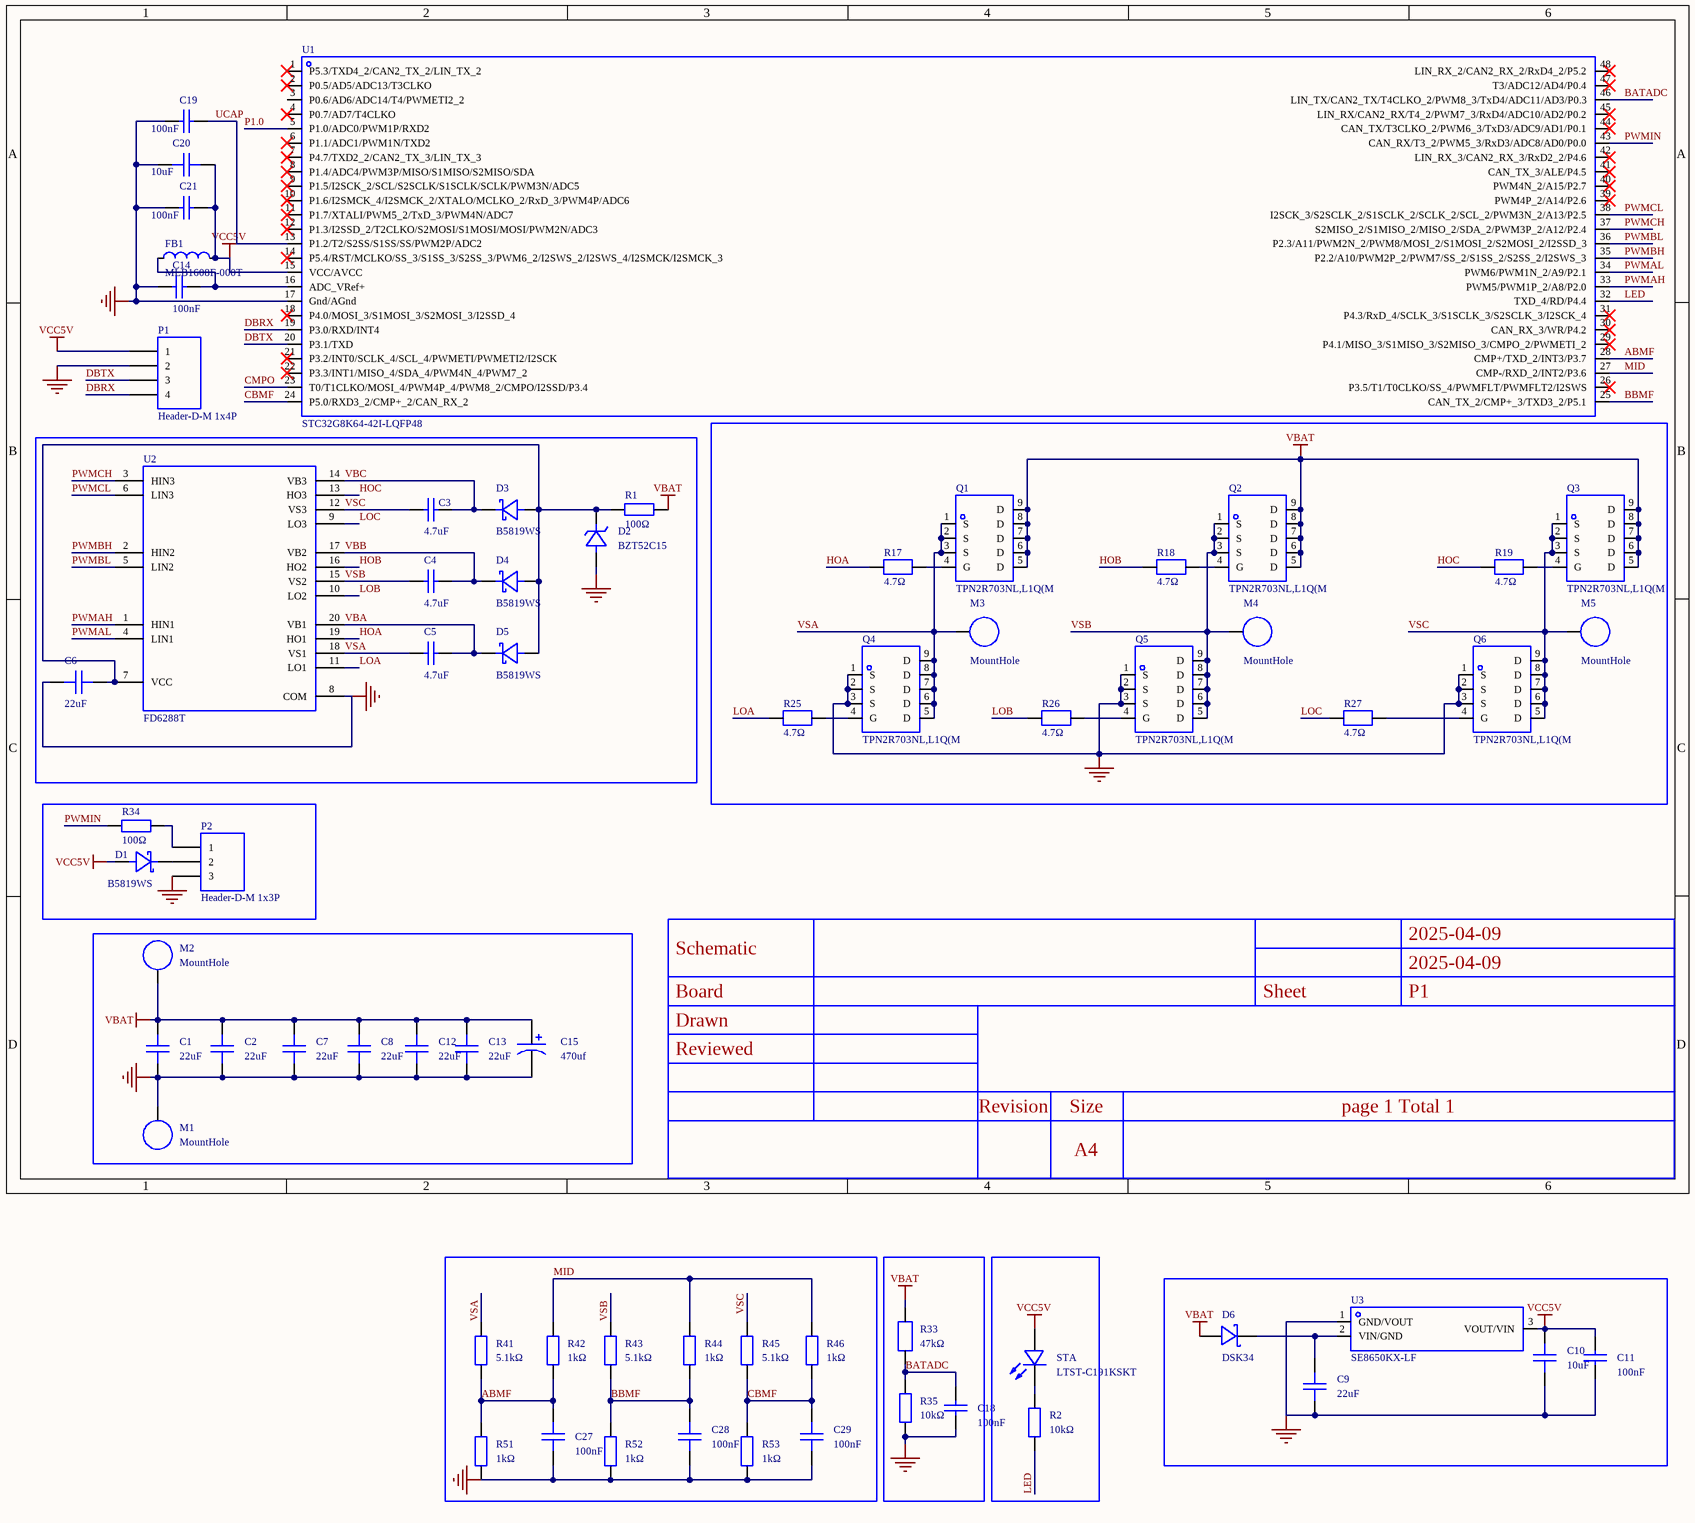
[diagram p0: MISC52085-3.schdoc]
# Altium project MISC52085-2.PrjPcb
1 sheet, 66 parts. Net scope: global (net labels, ports and power ports of the same name join across sheets).
Board file: MISC52085.pcbdoc

## Sheet MISC52085-3.schdoc
size 297 x 209 mm; Version: V1.0; @Project Name: MISC52085; @Page Count: 1; @Update Date: 2025-04-09; @Create Date: 2025-04-09; @Schematic Name: MISC52085; @Page No: 1; @Create Time: 14:04:51; @Update Time: 14:05:14; @Board Name: MISC52085

### Parts
C1  22uF  [C0805]
C2  22uF  [C0805]
C3  4.7uF  [C0805]
C4  4.7uF  [C0805]
C5  4.7uF  [C0805]
C6  22uF  [C0805]
C7  22uF  [C0805]
C8  22uF  [C0805]
C9  22uF  [C0805]
C10  10uF  [C0603]
C11  100nF  [C0603]
C12  22uF  [C0805]
C13  22uF  [C0805]
C14  100nF  [C0603]
C15  470uf  [焊盘]
C18  100nF  [C0603]
C19  100nF  [C0603]
C20  10uF  [C0603]
C21  100nF  [C0603]
C27  100nF  [C0402]
C28  100nF  [C0402]
C29  100nF  [C0402]
D1  B5819WS  [SOD-323_L1.7-W1.3-LS2.5-FD]
D2  BZT52C15  [SOD-123_L2.7-W1.6-LS3.7-RD]
D3  B5819WS  [SOD-323_L1.7-W1.3-LS2.5-FD]
D4  B5819WS  [SOD-323_L1.7-W1.3-LS2.5-FD]
D5  B5819WS  [SOD-323_L1.7-W1.3-LS2.5-FD]
D6  DSK34  [SOD-123_L2.8-W1.8-LS3.7-RD]
FB1  MLB1608F-000T  [L0603]
M1  MountHole  [3*4焊盘]
M2  MountHole  [3*4焊盘]
M3  MountHole  [3*4焊盘]
M4  MountHole  [3*4焊盘]
M5  MountHole  [3*4焊盘]
P1  Header-D-M 1x4P  [调试端口2.54_1X4]
P2  Header-D-M 1x3P  [3P]
Q1  TPN2R703NL,L1Q(M  [TSON-8_L3.1-W3.1-P0.65-LS3.3-BL-EP]
Q2  TPN2R703NL,L1Q(M  [TSON-8_L3.1-W3.1-P0.65-LS3.3-BL-EP]
Q3  TPN2R703NL,L1Q(M  [TSON-8_L3.1-W3.1-P0.65-LS3.3-BL-EP]
Q4  TPN2R703NL,L1Q(M  [TSON-8_L3.1-W3.1-P0.65-LS3.3-BL-EP]
Q5  TPN2R703NL,L1Q(M  [TSON-8_L3.1-W3.1-P0.65-LS3.3-BL-EP]
Q6  TPN2R703NL,L1Q(M  [TSON-8_L3.1-W3.1-P0.65-LS3.3-BL-EP]
R1  100Ω  [R0603]
R2  10kΩ  [R0603]
R17  4.7Ω  [R0603]
R18  4.7Ω  [R0603]
R19  4.7Ω  [R0603]
R25  4.7Ω  [R0603]
R26  4.7Ω  [R0603]
R27  4.7Ω  [R0603]
R33  47kΩ  [R0603]
R34  100Ω  [R0603]
R35  10kΩ  [R0603]
R41  5.1kΩ  [R0603]
R42  1kΩ  [R0603]
R43  5.1kΩ  [R0603]
R44  1kΩ  [R0603]
R45  5.1kΩ  [R0603]
R46  1kΩ  [R0603]
R51  1kΩ  [R0603]
R52  1kΩ  [R0603]
R53  1kΩ  [R0603]
STA  LTST-C191KSKT  [LED0603-RD-YELLOW]
U1  STC32G8K64-42I-LQFP48  [LQFP-48_L7.0-W7.0-P0.50-LS9.0-BL]
U2  FD6288T  [TSSOP-20_L6.5-W4.4-P0.65-LS6.4-BL]
U3  SE8650KX-LF  [SOT-89-3_L4.3-W2.3-P1.50-LS4.3-BR]

### Nets
GND: C1.1 C2.1 C6.1 C7.1 C8.1 C9.1 C10.1 C11.1 C12.1 C13.1 C14.1 C15.2 C18.1 C19.1 C20.1 C21.1 C27.1 C28.1 C29.1 D2.2(A) M1.1 P1.2 P2.3 Q4.1(S) Q4.2(S) Q4.3(S) Q5.1(S) Q5.2(S) Q5.3(S) Q6.1(S) Q6.2(S) Q6.3(S) R35.1 R51.1 R52.1 R53.1 U1.17(Gnd/AGnd) U2.8(COM) U3.1(GND/VOUT)
VBAT: C1.2 C2.2 C7.2 C8.2 C12.2 C13.2 C15.1 D6.2(A) M2.1 Q1.5(D) Q1.6(D) Q1.7(D) Q1.8(D) Q1.9(D) Q2.5(D) Q2.6(D) Q2.7(D) Q2.8(D) Q2.9(D) Q3.5(D) Q3.6(D) Q3.7(D) Q3.8(D) Q3.9(D) R1.2 R33.2
VCC5V: C10.2 C11.2 C20.2 C21.2 D1.1(A) FB1.2 P1.1 STA.2(+) U1.15(VCC/AVCC) U3.3(VOUT/VIN)
ABMF: C27.2 R41.1 R42.1 R51.2 U1.28(CMP+/TXD_2/INT3/P3.7)
BATADC: C18.2 R33.1 R35.2 U1.46(LIN_TX/CAN2_TX/T4CLKO_2/PWM8_3/TxD4/ADC11/AD3/P0.3)
BBMF: C28.2 R43.1 R44.1 R52.2 U1.25(CAN_TX_2/CMP+_3/TXD3_2/P5.1)
CBMF: C29.2 R45.1 R46.1 R53.2 U1.24(P5.0/RXD3_2/CMP+_2/CAN_RX_2)
CMPO: U1.23(T0/T1CLKO/MOSI_4/PWM4P_4/PWM8_2/CMPO/I2SSD/P3.4)
DBRX: P1.4 U1.19(P3.0/RXD/INT4)
DBTX: P1.3 U1.20(P3.1/TXD)
HOA: R17.1 U2.19(HO1)
HOB: R18.1 U2.16(HO2)
HOC: R19.1 U2.13(HO3)
LED: R2.1 U1.32(TXD_4/RD/P4.4)
LOA: R25.1 U2.11(LO1)
LOB: R26.1 U2.10(LO2)
LOC: R27.1 U2.9(LO3)
MID: R42.2 R44.2 R46.2 U1.27(CMP-/RXD_2/INT2/P3.6)
P1.0: U1.5(P1.0/ADC0/PWM1P/RXD2)
PWMAH: U1.33(PWM5/PWM1P_2/A8/P2.0) U2.1(HIN1)
PWMAL: U1.34(PWM6/PWM1N_2/A9/P2.1) U2.4(LIN1)
PWMBH: U1.35(P2.2/A10/PWM2P_2/PWM7/SS_2/S1SS_2/S2SS_2/I2SWS_3) U2.2(HIN2)
PWMBL: U1.36(P2.3/A11/PWM2N_2/PWM8/MOSI_2/S1MOSI_2/S2MOSI_2/I2SSD_3) U2.5(LIN2)
PWMCH: U1.37(S2MISO_2/S1MISO_2/MISO_2/SDA_2/PWM3P_2/A12/P2.4) U2.3(HIN3)
PWMCL: U1.38(I2SCK_3/S2SCLK_2/S1SCLK_2/SCLK_2/SCL_2/PWM3N_2/A13/P2.5) U2.6(LIN3)
PWMIN: R34.1 U1.43(CAN_RX/T3_2/PWM5_3/RxD3/ADC8/AD0/P0.0)
UCAP: C19.2 U1.13(P1.2/T2/S2SS/S1SS/SS/PWM2P/ADC2)
VBA: C5.2 D5.2(K) U2.20(VB1)
VBB: C4.2 D4.2(K) U2.17(VB2)
VBC: C3.2 D3.2(K) U2.14(VB3)
VSA: C5.1 M3.1 Q1.1(S) Q1.2(S) Q1.3(S) Q4.5(D) Q4.6(D) Q4.7(D) Q4.8(D) Q4.9(D) R41.2 U2.18(VS1)
VSB: C4.1 M4.1 Q2.1(S) Q2.2(S) Q2.3(S) Q5.5(D) Q5.6(D) Q5.7(D) Q5.8(D) Q5.9(D) R43.2 U2.15(VS2)
VSC: C3.1 M5.1 Q3.1(S) Q3.2(S) Q3.3(S) Q6.5(D) Q6.6(D) Q6.7(D) Q6.8(D) Q6.9(D) R45.2 U2.12(VS3)
NetC6_2: C6.2 D2.1(K) D3.1(A) D4.1(A) D5.1(A) R1.1 U2.7(VCC)
NetC9_2: C9.2 D6.1(K) U3.2(VIN/GND)
NetC14_2: C14.2 FB1.1 U1.16(ADC_VRef+)
NetD1_2: D1.2(K) P2.2
NetP2_1: P2.1 R34.2
NetQ1_4: Q1.4(G) R17.2
NetQ2_4: Q2.4(G) R18.2
NetQ3_4: Q3.4(G) R19.2
NetQ4_4: Q4.4(G) R25.2
NetQ5_4: Q5.4(G) R26.2
NetQ6_4: Q6.4(G) R27.2
NetR2_2: R2.2 STA.1(-)

Not connected (* = marked no-connect by the designer): U1 1(P5.3/TXD4_2/CAN2_TX_2/LIN_TX_2)* 2(P0.5/AD5/ADC13/T3CLKO)* 3(P0.6/AD6/ADC14/T4/PWMETI2_2) 4(P0.7/AD7/T4CLKO)* 6(P1.1/ADC1/PWM1N/TXD2)* 7(P4.7/TXD2_2/CAN2_TX_3/LIN_TX_3)* 8(P1.4/ADC4/PWM3P/MISO/S1MISO/S2MISO/SDA)* 9(P1.5/I2SCK_2/SCL/S2SCLK/S1SCLK/SCLK/PWM3N/ADC5)* 10(P1.6/I2SMCK_4/I2SMCK_2/XTALO/MCLKO_2/RxD_3/PWM4P/ADC6)* 11(P1.7/XTALI/PWM5_2/TxD_3/PWM4N/ADC7)* 12(P1.3/I2SSD_2/T2CLKO/S2MOSI/S1MOSI/MOSI/PWM2N/ADC3)* 14(P5.4/RST/MCLKO/SS_3/S1SS_3/S2SS_3/PWM6_2/I2SWS_2/I2SWS_4/I2SMCK/I2SMCK_3)* 18(P4.0/MOSI_3/S1MOSI_3/S2MOSI_3/I2SSD_4)* 21(P3.2/INT0/SCLK_4/SCL_4/PWMETI/PWMETI2/I2SCK)* 22(P3.3/INT1/MISO_4/SDA_4/PWM4N_4/PWM7_2)* 26(P3.5/T1/T0CLKO/SS_4/PWMFLT/PWMFLT2/I2SWS)* 29(P4.1/MISO_3/S1MISO_3/S2MISO_3/CMPO_2/PWMETI_2)* 30(CAN_RX_3/WR/P4.2)* 31(P4.3/RxD_4/SCLK_3/S1SCLK_3/S2SCLK_3/I2SCK_4)* 39(PWM4P_2/A14/P2.6)* 40(PWM4N_2/A15/P2.7)* 41(CAN_TX_3/ALE/P4.5)* 42(LIN_RX_3/CAN2_RX_3/RxD2_2/P4.6)* 44(CAN_TX/T3CLKO_2/PWM6_3/TxD3/ADC9/AD1/P0.1)* 45(LIN_RX/CAN2_RX/T4_2/PWM7_3/RxD4/ADC10/AD2/P0.2)* 47(T3/ADC12/AD4/P0.4)* 48(LIN_RX_2/CAN2_RX_2/RxD4_2/P5.2)*

### Notes on the sheet
- 2025-04-09
- Schematic
- Board
- Sheet
- P1
- Drawn
- Reviewed
- Revision
- Size
- A4
- page 1 Total 1

### Library data of the parts
C1 C2 C6-C9 C12 C13 = CL21A226MAQNNNE: Capacitance:22uF;Tolerance:±20%;Rated voltage:25V;Dielectric (temp. coefficient):X5R;; Manufacturer: SAMSUNG(三星); AddInBom: yes; ModelId: 1ba041120af144c991958decab20d241; ModelName: C0805_L2.0-W1.3-H1.3; ModelTransform: 78.74,51.181,0,0,0,0,0,0.0005,0; Tolerance: ±20%; Voltage Rated: 25V; Temperature Coefficient: X5R; Symbol: CL21A226MAQNNNE; Device: CL21A226MAQNNNE; LCSC Part Name: 22uF ±20% 25V; SupplierPart: C45783; ManufacturerPart: CL21A226MAQNNNE; Supplier Footprint: 0805; JLCPCB Part Class: Basic library; Datasheet: https://atta.szlcsc.com/upload/public/pdf/source/20160218/1457707763339.pdf; Supplier: LCSC; ConvertToPcb: yes; FootprintName: C0805; Value: 22uF
C3-C5 = CL21A475KAQNNNE: Capacitance:4.7uF;Tolerance:±10%;Rated voltage:25V;Dielectric (temp. coefficient):X5R;; Manufacturer: SAMSUNG(三星); AddInBom: yes; ModelId: 1ba041120af144c991958decab20d241; ModelName: C0805_L2.0-W1.3-H1.3; ModelTransform: 78.74,51.181,0,0,0,0,0,0.0005,0; Tolerance: ±10%; Voltage Rated: 25V; Temperature Coefficient: X5R; Symbol: CL21A475KAQNNNE; Device: CL21A475KAQNNNE; LCSC Part Name: 4.7uF ±10% 25V; SupplierPart: C1779; ManufacturerPart: CL21A475KAQNNNE; Supplier Footprint: 0805; JLCPCB Part Class: Basic library; Datasheet: https://atta.szlcsc.com/upload/public/pdf/source/20160218/1457707763339.pdf; Supplier: LCSC; ConvertToPcb: yes; FootprintName: C0805; Value: 4.7uF
C10 C20 = CGA0603X5R106K100JT: Capacitance:10uF;Tolerance:±10%;Rated voltage:10V;Temperature coefficient:X5R;; Manufacturer: HRE(芯声); AddInBom: yes; ModelId: ac125912035d415993ca9572d50418b1; ModelName: C0603_L1.6-W0.8-H0.8; ModelTransform: 62.992,31.496,0,0,0,0,0,0,0; Tolerance: ±10%; Voltage Rating: 10V; Temperature Coefficient: X5R; Symbol: CGA0603X5R106K100JT; Device: CGA0603X5R106K100JT; LCSC Part Name: 10uF ±10% 10V; SupplierPart: C6119842; ManufacturerPart: CGA0603X5R106K100JT; Supplier Footprint: 0603; JLCPCB Part Class: Extended library; Supplier: LCSC; ConvertToPcb: yes; FootprintName: C0603; Value: 10uF
C11 C14 C18 C19 C21 = CL10B104KO8NNNC: Capacitance:100nF;Tolerance:±10%;Rated voltage:16V;Dielectric (temp. coefficient):X7R;; Manufacturer: SAMSUNG(三星); AddInBom: yes; ModelId: ac125912035d415993ca9572d50418b1; ModelName: C0603_L1.6-W0.8-H0.8; ModelTransform: 62.992,31.496,0,0,0,0,0,0,0; Tolerance: ±10%; Voltage Rated: 16V; Temperature Coefficient: X7R; Symbol: CL10B104KO8NNNC; Device: CL10B104KO8NNNC; LCSC Part Name: 100nF ±10% 16V; SupplierPart: C66501; ManufacturerPart: CL10B104KO8NNNC; Supplier Footprint: 0603; JLCPCB Part Class: Extended library; Datasheet: https://atta.szlcsc.com/upload/public/pdf/source/20160218/1457707763339.pdf; Supplier: LCSC; ConvertToPcb: yes; FootprintName: C0603; Value: 100nF
C15 = 470uf: ConvertToPcb: yes; Device: 470uf; AddInBom: yes; SymbolName: 470uf
C27-C29 = CL05B104KO5NNNC: Capacitance:100nF;Tolerance:±10%;Rated voltage:16V;Dielectric (temp. coefficient):X7R;; Manufacturer: SAMSUNG(三星); AddInBom: yes; ModelId: 36a51122f27c49738f86b3bfa98863e0; ModelName: C0402_L1.0-W0.5-H0.5; ModelTransform: 39.37,19.685,0,0,0,0,0,0,0; Tolerance: ±10%; Voltage Rated: 16V; Temperature Coefficient: X7R; Symbol: CL05B104KO5NNNC; Device: CL05B104KO5NNNC; LCSC Part Name: 100nF ±10% 16V; SupplierPart: C1525; ManufacturerPart: CL05B104KO5NNNC; Supplier Footprint: 0402; JLCPCB Part Class: Basic library; Datasheet: https://atta.szlcsc.com/upload/public/pdf/source/20160218/1457707763339.pdf; Supplier: LCSC; ConvertToPcb: yes; FootprintName: C0402; Value: 100nF
D1 D3-D5 = B5819WS_C7420331: Diode configuration:Single;Forward voltage(Vf):600mV@1.0A;DC reverse voltage(Vr):40V;Rectified current:1A;; Manufacturer: 宏迦橙; AddInBom: yes; ModelId: 0f2f330c645944df9245ac3c3fec3456; ModelTransform: 98.425,49.2125,0,180,0,0,0,0,0; Diode Configuration: Single; Reverse Voltage (Vr): 40V; Rectified Current: 1A; Reverse Leakage Current (Ir): 1mA@40V; Symbol: B5819WS_C7420331; Device: B5819WS_C7420331; LCSC Part Name: 电压:40V 电流:1A; SupplierPart: C7420331; ManufacturerPart: B5819WS; Supplier Footprint: SOD-323; JLCPCB Part Class: Extended library; Datasheet: https://atta.szlcsc.com/upload/public/pdf/source/20230828/03CA0F4F90DAE368A7153B7B5E4D0651.pdf; Supplier: LCSC; ConvertToPcb: yes; FootprintName: SOD-323_L1.7-W1.3-LS2.5-FD; ModelName: SOD-323_L1.7-W1.3-LS2.5-FD; Forward Voltage (Vf@If): 600mV@1.0A
D2 = BZT52C15_C19077412: Diode configuration:Single;Zener voltage (nominal):15V;Zener voltage (range):14.25V~15.75V;Power dissipation(Pd):500mW;; Manufacturer: 宏嘉诚; AddInBom: yes; ModelId: ad7e39f9e5534b3c96ffdc5532ebb493; ModelName: SOD-123_L2.7-W1.6-H1.4-LS3.7; ModelTransform: 146.026,62.992,0,180,0,0,0.0005,0,0; Diode Configuration: Single; Zener Voltage(Nom): 15V; Reverse Leakage Current (Ir): 100nA@10.5V; Pd - Power Dissipation(Pd): 500mW; Impedance(Zzt): 40Ω; Symbol: BZT52C15_C19077412; Device: BZT52C15_C19077412; LCSC Part Name: BZT52C15; SupplierPart: C19077412; ManufacturerPart: BZT52C15; Supplier Footprint: SOD-123; JLCPCB Part Class: Extended library; Datasheet: https://atta.szlcsc.com/upload/public/pdf/source/20250106/E12AA82D484C9C66E469D005F460C1F7.pdf; Supplier: LCSC; ConvertToPcb: yes; FootprintName: SOD-123_L2.7-W1.6-LS3.7-RD; Zener Voltage(Range): 14.25V~15.75V
D6 = DSK34_C41029: Diode configuration:Single;Forward voltage(Vf):550mV@3A;DC reverse voltage(Vr):40V;Rectified current:3A;; Manufacturer: MDD(辰达半导体); AddInBom: yes; ModelId: 7884390a25fb4c08947731ebfba7e3f8; ModelTransform: 144.8816,62.992,0,0,0,0,0,0,0; Diode Configuration: Single; Reverse Voltage (Vr): 40V; Rectified Current: 3A; Reverse Leakage Current (Ir): 500uA@40V; Symbol: DSK34; Device: DSK34_C41029; LCSC Part Name: 电压:40V 电流:3A; SupplierPart: C41029; ManufacturerPart: DSK34; Supplier Footprint: SOD-123FL; JLCPCB Part Class: Extended library; Datasheet: https://atta.szlcsc.com/upload/public/pdf/source/20240710/931B7979AEEE628A0AE48522F9F6A0BB.pdf; Supplier: LCSC; ConvertToPcb: yes; FootprintName: SOD-123_L2.8-W1.8-LS3.7-RD; ModelName: SOD-123_L2.8-W1.8-LS3.7-RD; Forward Voltage (Vf@If): 550mV@3A
FB1 = MLB1608F-000T: Impedance@frequency:0Ω@100MHz;Tolerance:±25%;DC resistance(DCR):-;; Manufacturer: MetalLions(美铼); AddInBom: yes; ModelId: 2bc5ec593d464d6ba9807aec0b5673c2; ModelName: L0603_L1.6-W0.8-H0.5_BEAD; ModelTransform: 62.992,31.496,0,180,0,0,0.094,0.629,0; Tolerance: ±25%; Number of Circuits: 1; Symbol: MLB1608F-000T; Device: MLB1608F-000T; LCSC Part Name: 单路 0603磁珠 阻抗0Ω@100MHz; SupplierPart: C2844549; ManufacturerPart: MLB1608F-000T; Supplier Footprint: 0603; JLCPCB Part Class: Extended library; Datasheet: https://atta.szlcsc.com/upload/public/pdf/source/20230602/7F9B6FFD64AF4C161BE293D8440B9AF6.pdf; Supplier: LCSC; ConvertToPcb: yes; FootprintName: L0603; Impedance @ Frequency: 0Ω@100MHz; DC Resistance(DCR): -; Current Rating: -
M1-M5 = MountHole: Mounting hole; AddInBom: yes; Device: MountHole; Footprint Name: M3-MountHole-Plated-D6; ConvertToPcb: yes; SymbolName: MountHole
P1 = Header-D-M 1x4P: 1x4pin, through-hole, pin header; AddInBom: yes; Device: Header-D-M 1x4P; Revision: V1.0; Value: Header-D-M 1x4P; Footprint Name: HDR1X4-M; ConvertToPcb: yes; SymbolName: Header-D-M 1x4P
P2 = Header-D-M 1x3P: 1x3pin, through-hole, pin header; AddInBom: yes; Device: Header-D-M 1x3P; Revision: V1.0; Value: Header-D-M 1x3P; Footprint Name: HDR1X3-M; ConvertToPcb: yes; SymbolName: Header-D-M 1x3P
Q1-Q6 = TPN2R703NL,L1Q(M: Type:1 N-channel;Drain-source voltage(Vdss):30V;Continuous drain current(Id):-;On-resistance(RDS(on)@Vgs,Id):3.3mΩ@4.5V,22.5A;Power:42W;Threshold voltage(Vgs(th)@Id):1.3V@0.3mA;; Manufacturer: TOSHIBA(东芝); AddInBom: yes; ModelId: 054ae61349db4ab4a59bf8617c283080; ModelName: TSON-8_L3.1-W3.1-H0.9-P0.65-LS3.3-BL-EP; ModelTransform: 129.921,122.8344,0,90,0,0,0,0,0; Drain Source Voltage (Vdss): 30V; Power Dissipation (Pd): 42W; Input Capacitance (Ciss@Vds): 1.6nF@15V; Reverse Transfer Capacitance (Crss@Vds): 53pF@15V; Symbol: TPN2R703NL,L1Q(M; Device: TPN2R703NL,L1Q(M; LCSC Part Name: TPN2R703NL,L1Q(M; SupplierPart: C5307666; ManufacturerPart: TPN2R703NL,L1Q(M; Supplier Footprint: TSON-8; JLCPCB Part Class: Extended library; Datasheet: https://atta.szlcsc.com/upload/public/pdf/source/20221207/F3F28B90115C5E074AC0CD2ED28456D7.pdf; Supplier: LCSC; ConvertToPcb: yes; FootprintName: TSON-8_L3.1-W3.1-P0.65-LS3.3-BL-EP; Type: 1 N-channel; Continuous Drain Current (Id): -; Drain Source On Resistance (RDS(on)@Vgs,Id): 3.3mΩ@4.5V,22.5A; Gate Threshold Voltage (Vgs(th)@Id): 1.3V@0.3mA; Total Gate Charge (Qg@Vgs): -; Operating Temperature: -; Configuration: -
R1 R34 = 0603WAF1000T5E: Resistor type:Thick film resistor;Resistance:100Ω;Tolerance:±1%;Power:100mW;Max working voltage:75V;Temperature coefficient:±200ppm/℃;; Manufacturer: UNI-ROYAL(厚声); AddInBom: yes; ModelId: fc143cca1e79419f9cd78b61e9279f08; ModelTransform: 31.8897,63.7794,0,90,0,0,0,0,0; Tolerance: ±1%; Power(Watts): 100mW; Overload Voltage (Max): 75V; Symbol: 0603WAF1000T5E; Device: 0603WAF1000T5E; LCSC Part Name: 100Ω ±1% 100mW 厚膜电阻; SupplierPart: C22775; ManufacturerPart: 0603WAF1000T5E; Supplier Footprint: 0603; JLCPCB Part Class: Basic library; Datasheet: https://atta.szlcsc.com/upload/public/pdf/source/20200306/C422600_1E6D84923E4A46A82E41ADD87F860B5C.pdf; Supplier: LCSC; ConvertToPcb: yes; FootprintName: R0603; ModelName: R0603; Type: Thick film resistor; Value: 100Ω; Temperature Coefficient: ±200ppm/℃; Operating Temperature Range: -55℃~+155℃
R2 R35 = 0603WAF1002T5E: Resistor type:Thick film resistor;Resistance:10kΩ;Tolerance:±1%;Power:100mW;Max working voltage:75V;Temperature coefficient:±100ppm/℃;; Manufacturer: UNI-ROYAL(厚声); AddInBom: yes; ModelId: fc143cca1e79419f9cd78b61e9279f08; ModelTransform: 31.8897,63.7794,0,90,0,0,0,0,0; Tolerance: ±1%; Power(Watts): 100mW; Overload Voltage (Max): 75V; Symbol: 0603WAF1002T5E; Device: 0603WAF1002T5E; LCSC Part Name: 厚膜电阻 10kΩ ±1% 100mW; SupplierPart: C25804; ManufacturerPart: 0603WAF1002T5E; Supplier Footprint: 0603; JLCPCB Part Class: Basic library; Datasheet: https://atta.szlcsc.com/upload/public/pdf/source/20200306/C422600_1E6D84923E4A46A82E41ADD87F860B5C.pdf; Supplier: LCSC; ConvertToPcb: yes; FootprintName: R0603; ModelName: R0603; Type: Thick film resistor; Value: 10kΩ; Temperature Coefficient: ±100ppm/℃; Operating Temperature Range: -55℃~+155℃
R17-R19 R25-R27 = FRC0603J4R7 TS: Resistor type:Thick film resistor;Resistance:4.7Ω;Tolerance:±5%;Power:100mW;Working voltage:75V;Temperature coefficient:±200ppm/℃;; Manufacturer: FOJAN(富捷); AddInBom: yes; ModelId: fc143cca1e79419f9cd78b61e9279f08; ModelTransform: 31.8897,63.7794,0,90,0,0,0,0,0; Tolerance: ±5%; Power(Watts): 100mW; Voltage-Supply(Max): 75V; Symbol: FRC0603J4R7 TS; Device: FRC0603J4R7 TS; LCSC Part Name: 4.7Ω ±5% 100mW 厚膜电阻; SupplierPart: C2907168; ManufacturerPart: FRC0603J4R7 TS; Supplier Footprint: 0603; JLCPCB Part Class: Extended library; Datasheet: https://atta.szlcsc.com/upload/public/pdf/source/20211221/925EC7D7225764EE0046F22065062C87.pdf; Supplier: LCSC; ConvertToPcb: yes; FootprintName: R0603; ModelName: R0603; Type: Thick film resistor; Value: 4.7Ω; Temperature Coefficient: ±200ppm/℃; Operating Temperature: -55℃~+155℃
R33 = FRC0603F4702TS: Resistor type:Thick film resistor;Resistance:47kΩ;Tolerance:±1%;Power:100mW;Max working voltage:75V;Temperature coefficient:±100ppm/℃;; Manufacturer: FOJAN(富捷); AddInBom: yes; ModelId: fc143cca1e79419f9cd78b61e9279f08; ModelTransform: 31.8897,63.7794,0,90,0,0,0,0,0; Tolerance: ±1%; Power(Watts): 100mW; Overload Voltage (Max): 75V; Symbol: FRC0603F4702TS; Device: FRC0603F4702TS; LCSC Part Name: 47kΩ ±1% 100mW 厚膜电阻; SupplierPart: C2907042; ManufacturerPart: FRC0603F4702TS; Supplier Footprint: 0603; JLCPCB Part Class: Extended library; Datasheet: https://atta.szlcsc.com/upload/public/pdf/source/20211221/925EC7D7225764EE0046F22065062C87.pdf; Supplier: LCSC; ConvertToPcb: yes; FootprintName: R0603; ModelName: R0603; Type: Thick film resistor; Value: 47kΩ; Temperature Coefficient: ±100ppm/℃; Operating Temperature Range: -55℃~+155℃
R41 R43 R45 = 0603WAF5101T5E: Resistor type:Thick film resistor;Resistance:5.1kΩ;Tolerance:±1%;Power:100mW;Max working voltage:75V;Temperature coefficient:±100ppm/℃;; Manufacturer: UNI-ROYAL(厚声); AddInBom: yes; ModelId: fc143cca1e79419f9cd78b61e9279f08; ModelTransform: 31.8897,63.7794,0,90,0,0,0,0,0; Tolerance: ±1%; Power(Watts): 100mW; Overload Voltage (Max): 75V; Symbol: 0603WAF5101T5E; Device: 0603WAF5101T5E; LCSC Part Name: 5.1kΩ ±1% 100mW 厚膜电阻; SupplierPart: C23186; ManufacturerPart: 0603WAF5101T5E; Supplier Footprint: 0603; JLCPCB Part Class: Basic library; Datasheet: https://atta.szlcsc.com/upload/public/pdf/source/20200306/C422600_1E6D84923E4A46A82E41ADD87F860B5C.pdf; Supplier: LCSC; ConvertToPcb: yes; FootprintName: R0603; ModelName: R0603; Type: Thick film resistor; Value: 5.1kΩ; Temperature Coefficient: ±100ppm/℃; Operating Temperature Range: -55℃~+155℃
R42 R44 R46 R51-R53 = 0603WAF1001T5E: Resistor type:Thick film resistor;Resistance:1kΩ;Tolerance:±1%;Power:100mW;Max working voltage:75V;Temperature coefficient:±100ppm/℃;; Manufacturer: UNI-ROYAL(厚声); AddInBom: yes; ModelId: fc143cca1e79419f9cd78b61e9279f08; ModelTransform: 31.8897,63.7794,0,90,0,0,0,0,0; Tolerance: ±1%; Power(Watts): 100mW; Overload Voltage (Max): 75V; Symbol: 0603WAF1001T5E; Device: 0603WAF1001T5E; LCSC Part Name: 1kΩ ±1% 100mW 厚膜电阻; SupplierPart: C21190; ManufacturerPart: 0603WAF1001T5E; Supplier Footprint: 0603; JLCPCB Part Class: Basic library; Datasheet: https://atta.szlcsc.com/upload/public/pdf/source/20200306/C422600_1E6D84923E4A46A82E41ADD87F860B5C.pdf; Supplier: LCSC; ConvertToPcb: yes; FootprintName: R0603; ModelName: R0603; Type: Thick film resistor; Value: 1kΩ; Temperature Coefficient: ±100ppm/℃; Operating Temperature Range: -55℃~+155℃
STA = LTST-C191KSKT: Emitted color:Yellow;Forward voltage(VF):2.1V;Power:75mW;Forward current:20mA;Dominant wavelength:584.5nm~597nm;Diode configuration:-;Lens color:Colorless transparent lens;Color temperature:-;Luminous intensity:104mcd;Viewing angle:130°;Packaging:-;Operating temperature:-55℃~+85℃;; Manufacturer: LITEON(光宝); AddInBom: yes; ModelId: a8fc7d5425514cf49dd600af0a7bb223; ModelTransform: 63.7794,32.283,0,0,0,0,-1.969,0,0; Emitted Color: Yellow; Forward Voltage (VF): 2.1V; Power Dissipation: 75mW; Forward Current: 20mA; Peak Wavelength: 588nm; Luminous Intensity: 104mcd; Viewing Angle: 130°; Symbol: LTST-C191KSKT; Device: LTST-C191KSKT; LCSC Part Name: 黄灯; SupplierPart: C125100; ManufacturerPart: LTST-C191KSKT; Supplier Footprint: 0603; JLCPCB Part Class: Extended library; Datasheet: https://atta.szlcsc.com/upload/public/pdf/source/20180129/C125100_15171877314981315871.pdf; Supplier: LCSC; ConvertToPcb: yes; FootprintName: LED0603-RD-YELLOW; ModelName: LED0603-RD-YELLOW; Dominant Wavelength: 584.5nm~597nm; Diode Configuration: -; Lens Color: Colorless transparent lens; Color Temperature: -; Mounting Sytle: -; Operating Temperature: -55℃~+85℃
U1 = STC32G8K64-42I-LQFP48: Manufacturer: STC(宏晶); AddInBom: yes; ModelId: 093be70396ff421eb2cdb946d5311efc; ModelName: LQFP-48_L7.0-W7.0-H1.4-LS9.0-P0.50; ModelTransform: 354.331,354.331,0,0,0,0,0,0,0; Symbol: STC32G8K64-42I-LQFP48; Device: STC32G8K64-42I-LQFP48; LCSC Part Name: STC32G8K64-42I-LQFP48; SupplierPart: C7419403; ManufacturerPart: STC32G8K64-42I-LQFP48; Supplier Footprint: LQFP-48(7x7); JLCPCB Part Class: Extended library; Supplier: LCSC; ConvertToPcb: yes; FootprintName: LQFP-48_L7.0-W7.0-P0.50-LS9.0-BL
U2 = FD6288T: Three independent half-bridge gate driver ICs; Manufacturer: Fortior Tech(峰岹); Symbol: FD6288; AddInBom: yes; ModelId: c491f68934b34c649df5890a1d97cd0f; ModelName: TSSOP-20_L6.5-W4.4-H1.0-LS6.4-P0.65; ModelTransform: 251.969,255.906,0,90,0,0,0.0005,0,0; Device: FD6288T; LCSC Part Name: FD6288T; SupplierPart: C97683; ManufacturerPart: FD6288T; Supplier Footprint: TSSOP-20; JLCPCB Part Class: Extended library; Datasheet: https://atta.szlcsc.com/upload/public/pdf/source/20241101/0E2856EB301EAFFED732065FB088D773.pdf; Supplier: LCSC; ConvertToPcb: yes; FootprintName: TSSOP-20_L6.5-W4.4-P0.65-LS6.4-BL
U3 = SE8650KX-LF: Manufacturer: null; ManufacturerPart: SE8650KX-LF-SOT89-3; ConvertToPcb: yes; Device: SE8650KX-LF; Supplier: LCSC; SupplierPart: C9900156618; AddInBom: yes; SymbolName: SE8650KX-LF; FootprintName: SOT-89-3_L4.3-W2.3-P1.50-LS4.3-BR